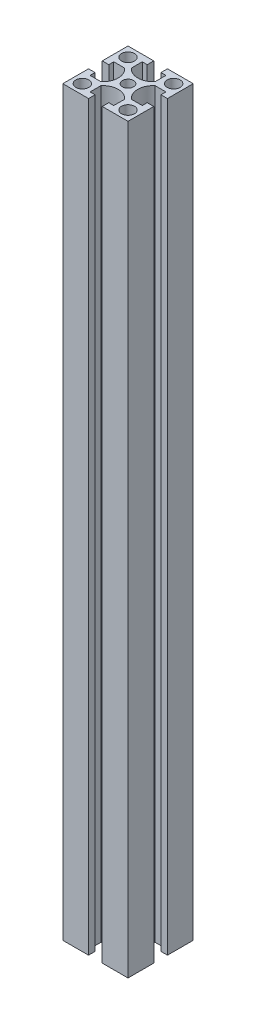
SolidWorks part; units mm, degrees
ref_plane "前视基准面" through (0, 0, 0) normal (0, 0, 1) x (1, 0, 0)
ref_plane "上视基准面" through (0, 0, 0) normal (0, 1, 0) x (1, 0, 0)
ref_plane "右视基准面" through (0, 0, 0) normal (1, 0, 0) x (0, 0, -1)
sketch "草图1" plane through (0, 0, 0) normal (0, 0, 1) x (1, 0, 0)
  line L0 (0, 0) -> (0, 455)
  dimension "D1" = 455
other "東野鋁型材 EF4040(1)"
ref_plane "基准面1" through (0, 0, 0) normal (0, 1, 0) x (-1, 0, 0)
sketch "草圖3" plane through (0, 0, 0) normal (0, 1, 0) x (-1, 0, 0)
  line L0 (-20, -20) -> (-4.2, -20)
  line L1 (-4.2, -20) -> (-4.2, -16)
  line L2 (-4.2, -16) -> (-7.25, -16)
  line L3 (-7.25, -16) -> (-7.25, -9.361)
  line L4 (7.25, -9.361) -> (7.25, -16)
  line L5 (7.25, -16) -> (4.2, -16)
  line L6 (4.2, -16) -> (4.2, -20)
  line L7 (4.2, -20) -> (20, -20)
  line L8 (20, -20) -> (20, -4.2)
  line L9 (20, -4.2) -> (16, -4.2)
  line L10 (16, -4.2) -> (16, -7.25)
  line L11 (16, -7.25) -> (9.361, -7.25)
  line L12 (9.361, 7.25) -> (16, 7.25)
  line L13 (16, 7.25) -> (16, 4.2)
  line L14 (16, 4.2) -> (20, 4.2)
  line L15 (20, 4.2) -> (20, 20)
  line L16 (20, 20) -> (4.2, 20)
  line L17 (4.2, 20) -> (4.2, 16)
  line L18 (4.2, 16) -> (7.25, 16)
  line L19 (7.25, 16) -> (7.25, 9.361)
  line L20 (-7.25, 9.361) -> (-7.25, 16)
  line L21 (-7.25, 16) -> (-4.2, 16)
  line L22 (-4.2, 16) -> (-4.2, 20)
  line L23 (-4.2, 20) -> (-20, 20)
  line L24 (-20, 20) -> (-20, 4.2)
  line L25 (-20, 4.2) -> (-16, 4.2)
  line L26 (-16, 4.2) -> (-16, 7.25)
  line L27 (-16, 7.25) -> (-9.361, 7.25)
  line L28 (-9.361, -7.25) -> (-16, -7.25)
  line L29 (-16, -7.25) -> (-16, -4.2)
  line L30 (-16, -4.2) -> (-20, -4.2)
  line L31 (-20, -4.2) -> (-20, -20)
  circle A0 centre (-14, -14) radius 4
  circle A1 centre (0, 0) radius 3.4
  circle A2 centre (14, -14) radius 4
  circle A3 centre (-14, 14) radius 4
  circle A4 centre (14, 14) radius 4
  arc A5 (7.25, -9.361) -> (-7.25, -9.361) centre (0, -15.5) ccw
  arc A6 (9.361, 7.25) -> (9.361, -7.25) centre (15.5, 0) ccw
  arc A7 (-7.25, 9.361) -> (7.25, 9.361) centre (0, 15.5) ccw
  arc A8 (-9.361, -7.25) -> (-9.361, 7.25) centre (-15.5, 0) ccw
  point P50 (0, 0)
